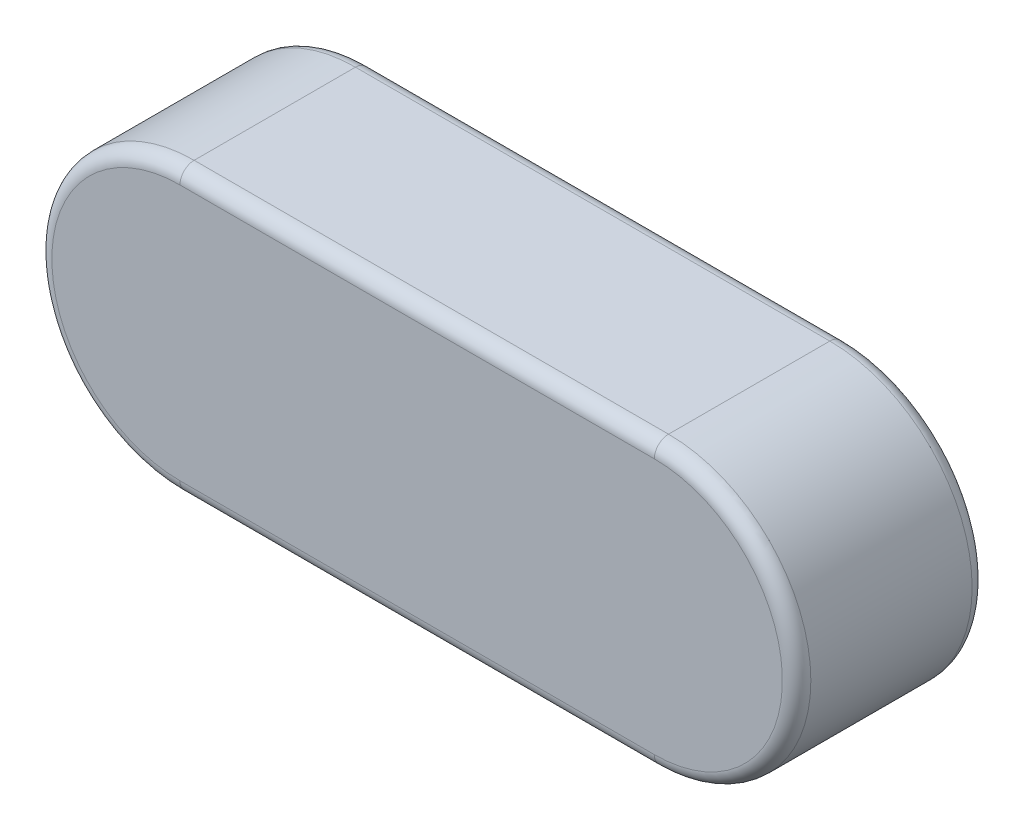
from build123d import *

# Parameters (mm, degrees)
EXTRUDE_523_DEPTH = 8
FILLET_1_R        = 0.6


with BuildPart() as part:
    # 草图1 → Extrude 523 (new body)
    with BuildSketch(Plane.XY):
        with BuildLine():
            Line((-10, 6), (10, 6))
            ThreePointArc((10, 6), (16, 0), (10, -6))
            Line((10, -6), (-10, -6))
            ThreePointArc((-10, -6), (-16, 0), (-10, 6))
        make_face()
    extrude(amount=EXTRUDE_523_DEPTH)

    # 圆角1
    fillet_1_edges = [part.edges().sort_by_distance(p)[0] for p in [
        (16, 0, 8),
        (0, 6, 8),
        (-16, 0, 8),
        (0, 6, 0),
        (16, 0, 0),
        (0, -6, 0),
        (-16, 0, 0),
        (0, -6, 8),
    ]]
    fillet(fillet_1_edges, radius=FILLET_1_R)


solid = part.part
